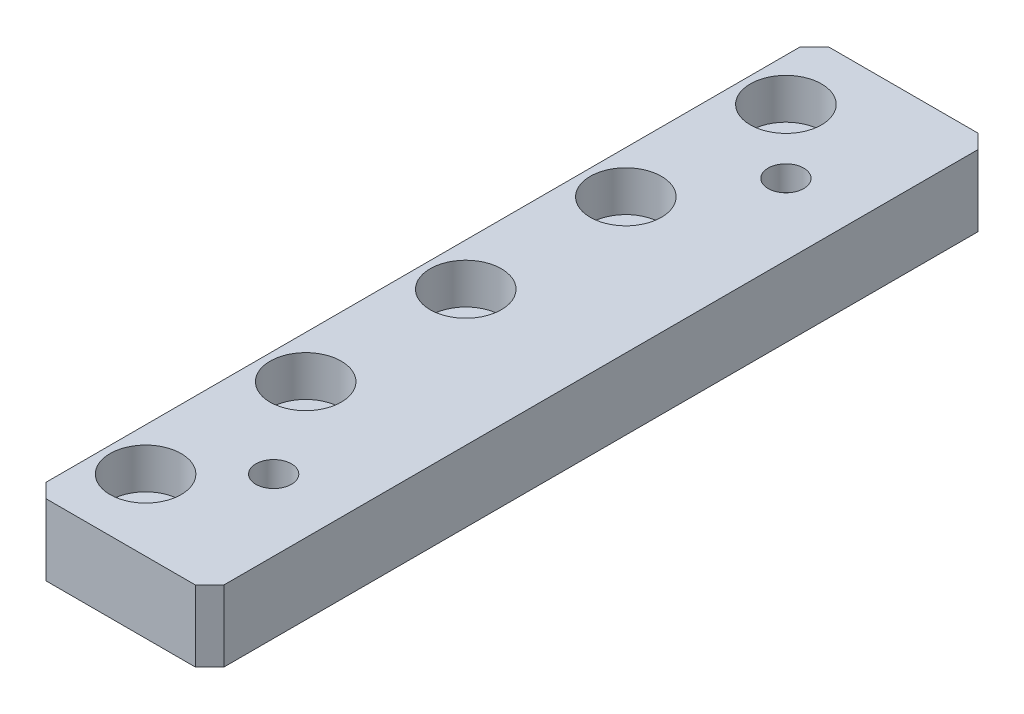
SolidWorks part; units mm, degrees
material "A6061 T6"
ref_plane "前视基准面" through (0, 0, 0) normal (0, 0, 1) x (1, 0, 0)
ref_plane "上视基准面" through (0, 0, 0) normal (0, 1, 0) x (1, 0, 0)
ref_plane "右视基准面" through (0, 0, 0) normal (1, 0, 0) x (0, 0, -1)
sketch "草图1" plane through (0, 0, 0) normal (0, 1, 0) x (1, 0, 0)
  line L1 (-12.5, 55) -> (12.5, 55)
  line L2 (-12.5, 55) -> (-12.5, -55)
  line L3 (-12.5, -55) -> (12.5, -55)
  line L4 (12.5, 55) -> (12.5, -55)
  line L5 (-12.5, 55) -> (12.5, -55) construction
  line L6 (-12.5, -55) -> (12.5, 55) construction
  point P0 (0, 0)
  dimension "D1" = 25
  dimension "D2" = 110
extrude "凸台-拉伸1" add sketch "草图1" along normal blind 10
chamfer "倒角1" distance 2 angle 45 4 edges at (-12.5, 5, -55) (12.5, 5, -55) (-12.5, 5, 55) (12.5, 5, 55)
hole_wizard "打孔尺寸(%根据)内六角圆柱头螺钉的类型1" positions "草图2" profile "草图3" counterbore size "M5" standard "GB"
sketch "草图2" plane through (0, 10, 0) normal (0, 1, 0) x (1, 0, 0)
  line L0 (-12.5, 53) -> (-12.5, -53) construction
  line L1 (-10.5, -55) -> (10.5, -55) construction
  point P0 (-6.5, -45)
  point P3 (-6.5, 0)
  point P14 (-6.5, 45)
  point P23 (-6.5, -22.5)
  point P25 (-6.5, 22.5)
  dimension "D1" = 6
  dimension "D2" = 10
  dimension "D3" = 45
  dimension "D4" = 45
  dimension "D5" = 45
  dimension "D6" = 22.5
sketch "草图3" plane through (-6.5, 10, 45) normal (1, 0, 0) x (0, 0, 1)
  line L0 (0, 0) -> (0, 14.0524)
  line L1 (0, 14.0524) -> (2.75, 12.4)
  line L2 (2.75, 12.4) -> (2.75, 5.7)
  line L3 (2.75, 5.7) -> (5, 5.7)
  line L4 (5, 5.7) -> (5, 0)
  line L5 (5, 0) -> (0, 0)
  line L10 (0, 14.0524) -> (-2.75, 12.4) construction
  line L11 (0, -6.35) -> (0, 107.95) construction
  dimension "孔直径" = 5.5
  dimension "孔深度" = 12.4
  dimension "柱形沉头孔直径" = 10
  dimension "柱形沉头孔深度" = 5.7
  dimension "导头角度" = 118
hole_wizard "打孔尺寸(%根据)内六角圆柱头螺钉的类型1" positions "草图4" profile "草图5" counterbore size "M3" standard "GB"
sketch "草图4" plane through (0, 0, 0) normal (0, -1, 0) x (-1, 0, 0)
  line L0 (-12.5, -53) -> (-12.5, 53) construction
  line L3 (0, 0) -> (-20.9862, 0) construction
  point P0 (-2.5, -36)
  point P2 (-2.5, 36)
  dimension "D1" = 10
  dimension "D2" = 72
sketch "草图5" plane through (2.5, 0, 36) normal (1, 0, 0) x (0, 0, -1)
  line L0 (0, 0) -> (0, 16.0215)
  line L1 (0, 16.0215) -> (1.7, 15)
  line L2 (1.7, 15) -> (1.7, 3.4)
  line L3 (1.7, 3.4) -> (3, 3.4)
  line L4 (3, 3.4) -> (3, 0)
  line L5 (3, 0) -> (0, 0)
  line L10 (0, 16.0215) -> (-1.7, 15) construction
  line L11 (0, -6.35) -> (0, 107.95) construction
  dimension "孔直径" = 3.4
  dimension "孔深度" = 15
  dimension "柱形沉头孔直径" = 6
  dimension "柱形沉头孔深度" = 3.4
  dimension "导头角度" = 118
sketch "草图6" plane through (0, 10, 0) normal (0, 1, 0) x (1, 0, 0)
  circle A0 centre (2.5, -36) radius 2.5
  circle A1 centre (2.5, 36) radius 2.5
  dimension "D1" = 5
extrude "切除-拉伸1" cut sketch "草图6" against normal blind 3.5
hole_wizard "M5 螺纹孔1" positions "草图7" profile "草图8" tap size "M5" standard "GB"
sketch "草图7" plane through (0, 10, 0) normal (0, 1, 0) x (1, 0, 0)
  point P0 (0, 0)
sketch "草图8" plane through (0, 10, 0) normal (1, 0, 0) x (0, 0, 1)
  line L0 (0, 0) -> (0, 16.2618)
  line L1 (0, 16.2618) -> (2.1, 15)
  line L2 (2.1, 15) -> (2.1, 0)
  line L5 (2.1, 0) -> (0, 0)
  line L10 (0, 16.2618) -> (-2.1, 15) construction
  line L11 (0, -6.35) -> (0, 107.95) construction
  dimension "螺纹孔钻头直径" = 4.2
  dimension "螺纹孔钻头深度" = 15
  dimension "导头角度" = 118
